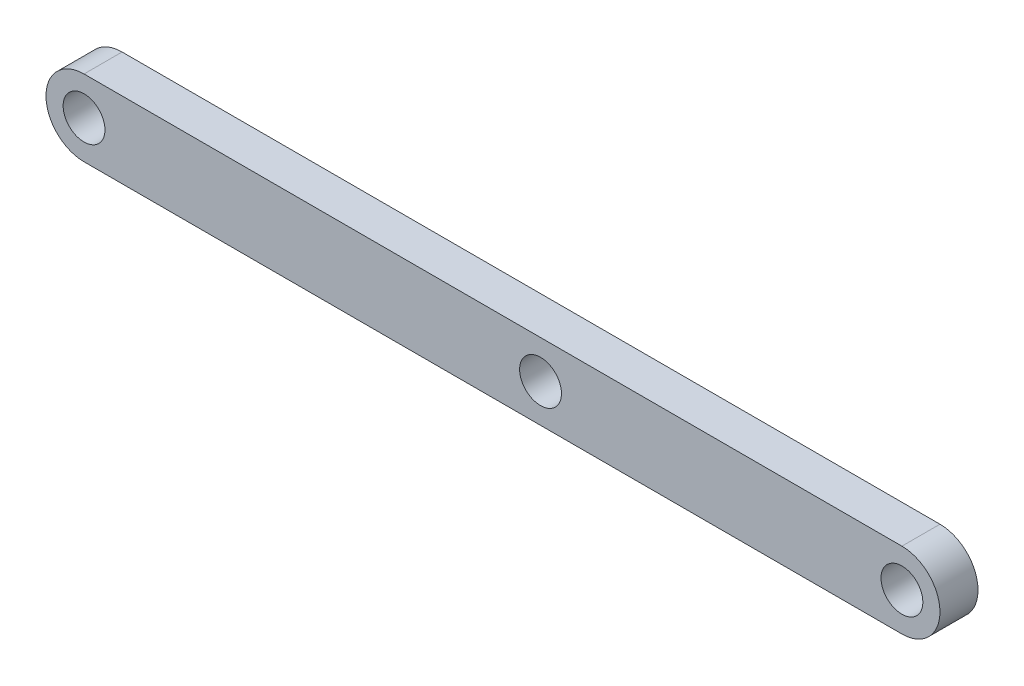
SolidWorks part; units mm, degrees
ref_plane "Alzado" through (0, 0, 0) normal (0, 0, 1) x (1, 0, 0)
ref_plane "Planta" through (0, 0, 0) normal (0, 1, 0) x (1, 0, 0)
ref_plane "Vista lateral" through (0, 0, 0) normal (1, 0, 0) x (0, 0, -1)
sketch "Sketch1" plane through (0, 0, 0) normal (0, 0, 1) x (1, 0, 0)
  line L0 (-10.75, 0) -> (10.75, 0) construction
  line L1 (-10.75, 1) -> (10.75, 1)
  line L2 (-10.75, -1) -> (10.75, -1)
  arc A0 (-10.75, 1) -> (-10.75, -1) centre (-10.75, 0) ccw
  arc A1 (10.75, -1) -> (10.75, 1) centre (10.75, 0) ccw
  circle A2 centre (-10.75, 0) radius 0.55
  circle A3 centre (10.75, 0) radius 0.55
  circle A4 centre (1.25, 0) radius 0.55
  point P3 (0, 0)
  dimension "D3" = 1.1
  dimension "D4" = 12
  dimension "D1" = 21.5
  dimension "D2" = 2
extrude "Thigh1 length" add sketch "Sketch1" along normal mid plane 1
sketch "Sketch2" plane through (0, 0, 0.5) normal (0, 0, 1) x (1, 0, 0)
  circle A0 centre (-10.75, 0) radius 1.8
  circle A1 centre (10.75, 0) radius 1.8
  dimension "D1" = 3.6
extrude "Cortar-Extruir1" [suppressed] cut sketch "Sketch2" against normal blind 1
